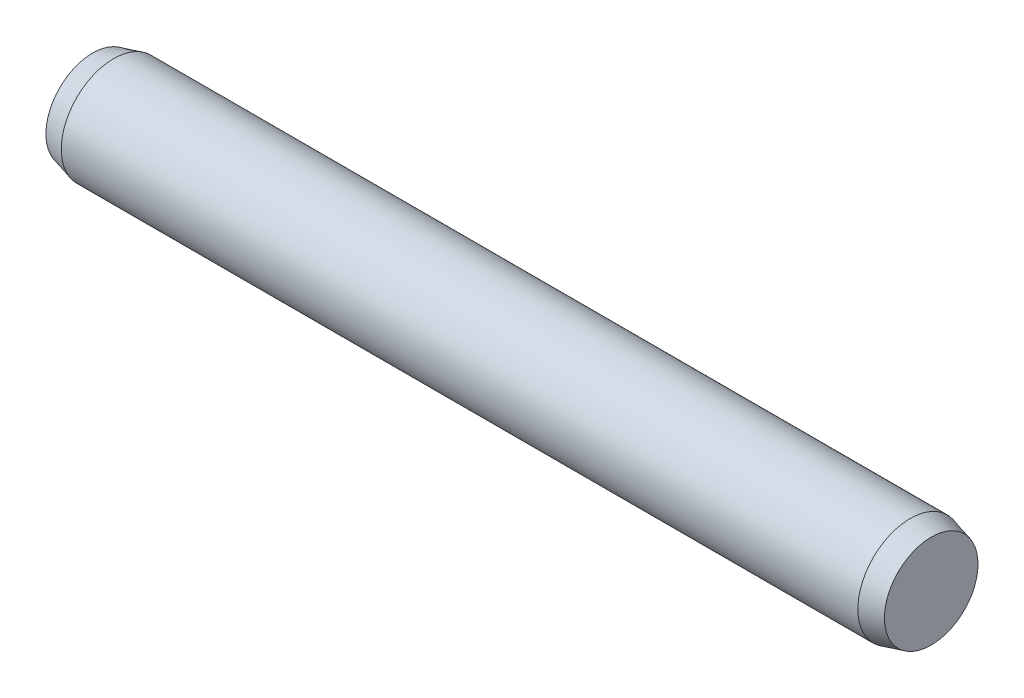
SolidWorks part; units mm, degrees
ref_plane "Front Plane" through (0, 0, 0) normal (0, 0, 1) x (1, 0, 0)
ref_plane "Top Plane" through (0, 0, 0) normal (0, 1, 0) x (1, 0, 0)
ref_plane "Right Plane" through (0, 0, 0) normal (1, 0, 0) x (0, 0, -1)
sketch "Dimensioned Sketch" plane through (0, 0, 0) normal (0, 0, 1) x (1, 0, 0)
  line L0 (0, 0) -> (-0.7681, 0) construction
  line L1 (0, 0) -> (80, 0)
  line L2 (2, 5) -> (78, 5)
  line L3 (80, 4.4641) -> (80, 0)
  line L4 (78, 5) -> (80, 4.4641)
  line L5 (2, -5) -> (78, -5) construction
  line L6 (2, 5) -> (0, 4.4641)
  line L7 (0, 4.4641) -> (0, 0)
  point P13 (40, 5)
  dimension "D1" = 165
  dimension "D2" = 2
  dimension "D3" = 165
  dimension "c" = 2
  dimension "l" = 80
  dimension "d" = 10
revolve "Base-Revolve" add sketch "Dimensioned Sketch" angle 360 about L0
